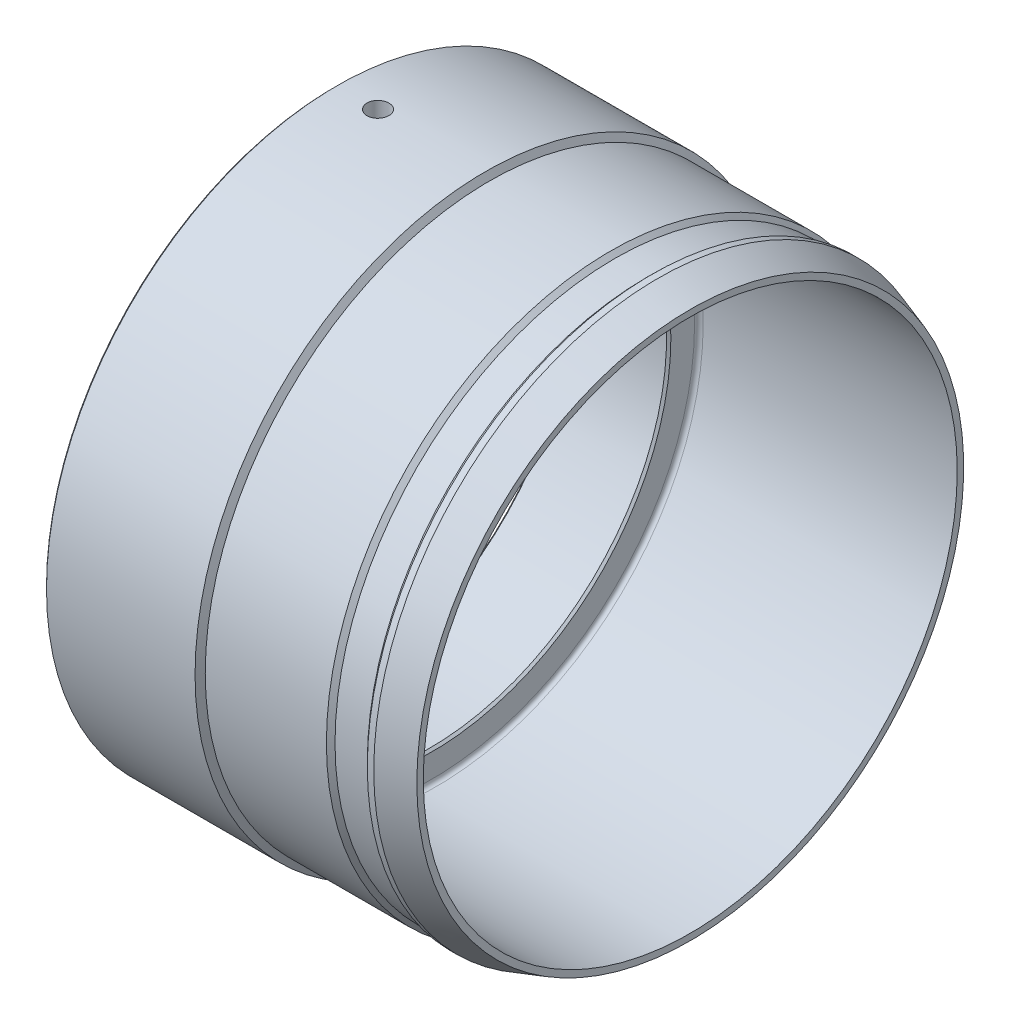
SolidWorks part; units mm, degrees
material "42CrMo"
ref_plane "Front Plane" through (0, 0, 0) normal (0, 0, 1) x (1, 0, 0)
ref_plane "Top Plane" through (0, 0, 0) normal (0, 1, 0) x (1, 0, 0)
ref_plane "Right Plane" through (0, 0, 0) normal (1, 0, 0) x (0, 0, -1)
sketch "Sketch1" plane through (0, 0, 0) normal (0, 0, 1) x (1, 0, 0)
  line L0 (0, 0) -> (796.1355, 0) construction
  line L1 (0, 0) -> (0, 577.9016) construction
  line L2 (0, 110) -> (45, 110)
  line L3 (165, 124) -> (165, 127)
  line L4 (165, 127) -> (150, 132)
  line L5 (150, 132) -> (147, 132)
  line L7 (145, 130) -> (130, 130)
  line L9 (128, 132) -> (71.7321, 132)
  line L10 (45, 110) -> (45, 124)
  line L11 (45, 124) -> (165, 124)
  line L12 (70, 135) -> (71.7321, 132)
  line L13 (130, 130) -> (128, 132)
  line L14 (145, 130) -> (147, 132)
  line L15 (70, 135) -> (0, 135)
  line L16 (0, 135) -> (0, 110)
  dimension "D1" = 165
  dimension "D2" = 110
  dimension "D3" = 25
  dimension "D4" = 20
  dimension "D5" = 70
  dimension "D6" = 15
  dimension "D7" = 8
  dimension "D8" = 8
  dimension "D9" = 45
  dimension "D10" = 2
  dimension "D11" = 130
  dimension "D12" = 124
  dimension "D13" = 3
  dimension "D14" = 120
revolve "Revolve1" add sketch "Sketch1" angle 360 about L0
fillet "Fillet1" radius 2 1 edges at (45, 0, 124)
chamfer "Chamfer1" distance 1 angle 45 3 edges at (45, 0, 110) (0, 0, 110) (0, 0, 135)
sketch "Sketch5" plane through (0, 0, 0) normal (0, 1, 0) x (1, 0, 0)
  line L0 (0, 0) -> (43.3022, 0) construction
  line L1 (0, 134) -> (0, -134) construction
sketch "Sketch7" plane through (0, 0, 0) normal (1, 0, 0) x (0, 0, -1)
  line L0 (0, 0) -> (0, 135) construction
  circle A0 centre (0, 0) radius 135 construction
sketch "Sketch8" plane through (0, 0, 0) normal (0, 0, 1) x (1, 0, 0)
  line L0 (1, 135) -> (70, 135) construction
  line L1 (70, 135) -> (70, -135) construction
hole_wizard "M12 Tapped Hole1" positions "3DSketch3" profile "Sketch9" tap size "M12" standard "GB" end condition through all
sketch3d "3DSketch3"
  line L0 (1, 135, 0) -> (70, 135, 0) construction
  point P5 (20, 135, 0)
  dimension "D1" = 20
sketch "Sketch9" plane through (20, 135, 0) normal (1, 0, 0) x (0, 0, 1)
  line L0 (0, 0) -> (0, 270)
  line L1 (0, 270) -> (5.1, 270)
  line L2 (5.1, 270) -> (5.1, 0)
  line L5 (5.1, 0) -> (0, 0)
  line L11 (0, -6.35) -> (0, 107.95) construction
  dimension "通孔螺纹孔钻头直径" = 10.2
  dimension "通孔螺纹孔钻头深度" = 270
cosmetic thread "CosmeticThread hole thread 4" parameters "D2"=12
